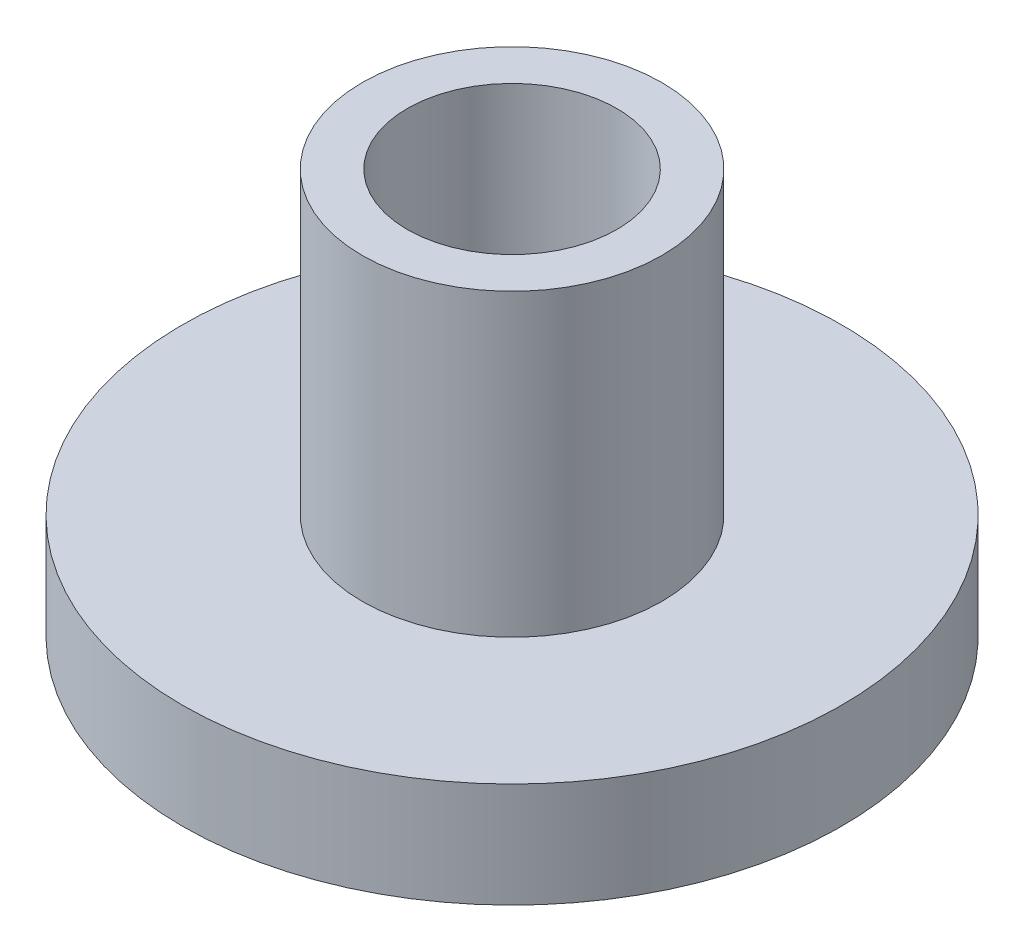
from build123d import *

# Parameters (mm, degrees)
SKETCH1_R             = 11
SKETCH1_R_2           = 5
BOSS_EXTRUDE1_DEPTH   = 3.5
SKETCH1_2_R           = 5
BOSS_EXTRUDE2_DEPTH   = 1.25
SKETCH1_3_R           = 5
BOSS_EXTRUDE3_DEPTH   = 13.5
M8X1_0_TAPPED_HOLE1_D = 7


with BuildPart() as part:
    # Sketch1 → Boss-Extrude1 (new body)
    with BuildSketch(Plane(origin=(0, 0, 0), x_dir=(1, 0, 0), z_dir=(0, 1, 0))):
        with Locations(Location((0, 0, 0), (0, 0, 270))):
            Circle(SKETCH1_R)
        with Locations(Location((0, 0, 0), (0, 0, 270))):
            Circle(SKETCH1_R_2, mode=Mode.SUBTRACT)
    extrude(amount=BOSS_EXTRUDE1_DEPTH)



with BuildPart() as body_2:
    # Sketch1<2> → Boss-Extrude2 (new body)
    with BuildSketch(Plane(origin=(0, 0, 0), x_dir=(1, 0, 0), z_dir=(0, 1, 0))):
        with Locations(Location((0, 0, 0), (0, 0, 270))):
            Circle(SKETCH1_2_R)
    extrude(amount=-BOSS_EXTRUDE2_DEPTH)


with BuildPart() as part_1:
    add(part.part)

    add(body_2.part)  # Boss-Extrude3 merges body 2
    # Sketch1<3> → Boss-Extrude3 (add)
    with BuildSketch(Plane(origin=(0, 0, 0), x_dir=(1, 0, 0), z_dir=(0, 1, 0))):
        with Locations(Location((0, 0, 0), (0, 0, 270))):
            Circle(SKETCH1_3_R)
    extrude(amount=BOSS_EXTRUDE3_DEPTH)

    # M8x1.0 Tapped Hole1 (through all)
    with Locations(Plane.ZX.offset(13.5)):
        with Locations((0, 0)):
            Hole(M8X1_0_TAPPED_HOLE1_D / 2)


solid = part_1.part
